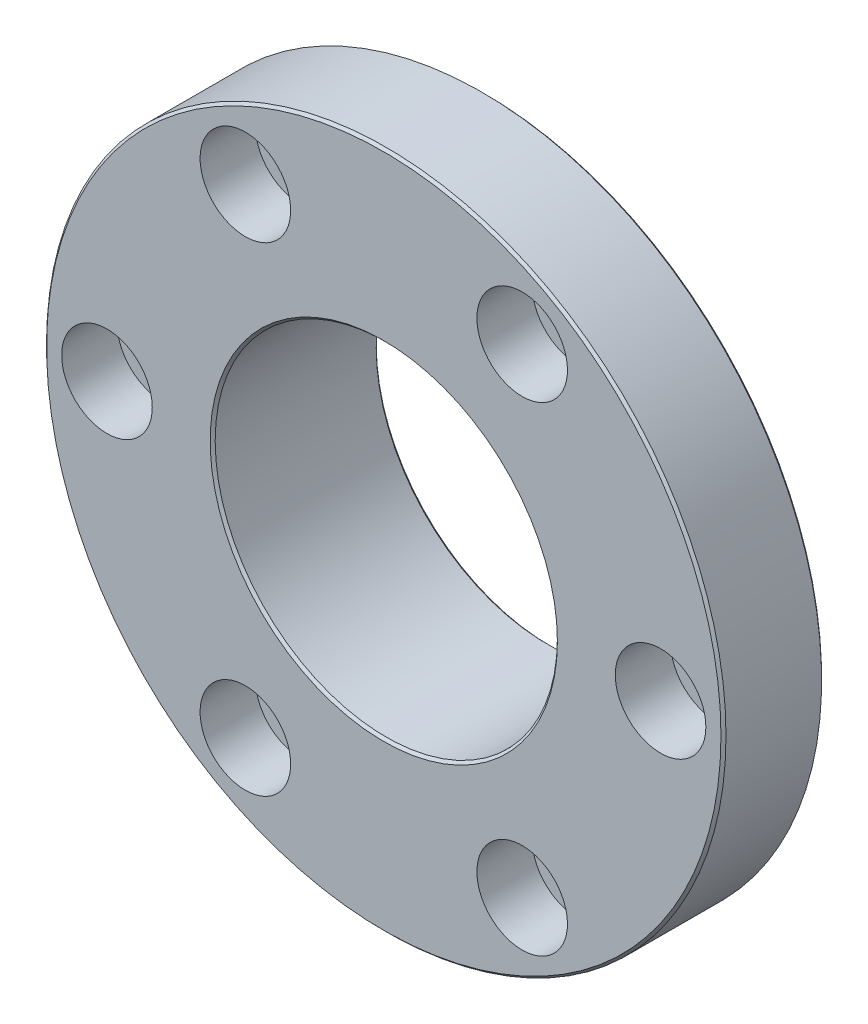
SolidWorks part; units mm, degrees
material "合金钢"
ref_plane "前视基准面" through (0, 0, 0) normal (0, 0, 1) x (1, 0, 0)
ref_plane "上视基准面" through (0, 0, 0) normal (0, 1, 0) x (1, 0, 0)
ref_plane "右视基准面" through (0, 0, 0) normal (1, 0, 0) x (0, 0, -1)
sketch "草图1" plane through (0, 0, 0) normal (0, 1, 0) x (1, 0, 0)
  line L0 (0, 0) -> (0, -62096.3984) construction
  line L1 (-34, 0) -> (-67.5, 0)
  line L2 (-67.5, 0) -> (-67.5, 20)
  line L3 (-67.5, 20) -> (-42.5, 20)
  line L4 (-42.5, 20) -> (-42.5, 33)
  line L5 (-42.5, 33) -> (-34, 33)
  line L6 (-34, 33) -> (-34, 0)
  dimension "D1" = 135
  dimension "D2" = 85
  dimension "D3" = 68
  dimension "D4" = 20
  dimension "D5" = 13
revolve "旋转1" add sketch "草图1" angle 360 about L0
hole_wizard "打孔尺寸(%根据)内六角圆柱头螺钉的类型1" positions "草图2" profile "草图3" counterbore size "M10" standard "GB" end condition through all
sketch "草图2" plane through (0, 0, 0) normal (0, 0, 1) x (1, 0, 0)
  circle A1 centre (0, 0) radius 67.5 construction
  point P0 (55, 0)
  dimension "D1" = 12.5
sketch "草图3" plane through (55, 0, 0) normal (1, 0, 0) x (0, -1, 0)
  line L0 (0, 0) -> (0, 33)
  line L1 (0, 33) -> (5.5, 33)
  line L3 (5.5, 33) -> (5.5, 11)
  line L4 (5.5, 11) -> (9, 11)
  line L5 (9, 11) -> (9, 0)
  line L7 (9, 0) -> (0, 0)
  line L11 (0, -6.35) -> (0, 107.95) construction
  dimension "通孔孔直径" = 11
  dimension "通孔孔深度" = 33
  dimension "柱形沉头孔直径" = 18
  dimension "柱形沉头孔深度" = 11
pattern_circular "阵列(圆周)1" count 6 over 360 about axis through (0, 0, 0) along (0, 0, 1) of "打孔尺寸(%根据)内六角圆柱头螺钉的类型1"
chamfer "倒角1" distance 0.5 angle 45 5 edges at (-34, 0, -33) (-42.5, 0, -33) (-67.5, 0, -20) (-34, 0, 0) (-67.5, 0, 0)
